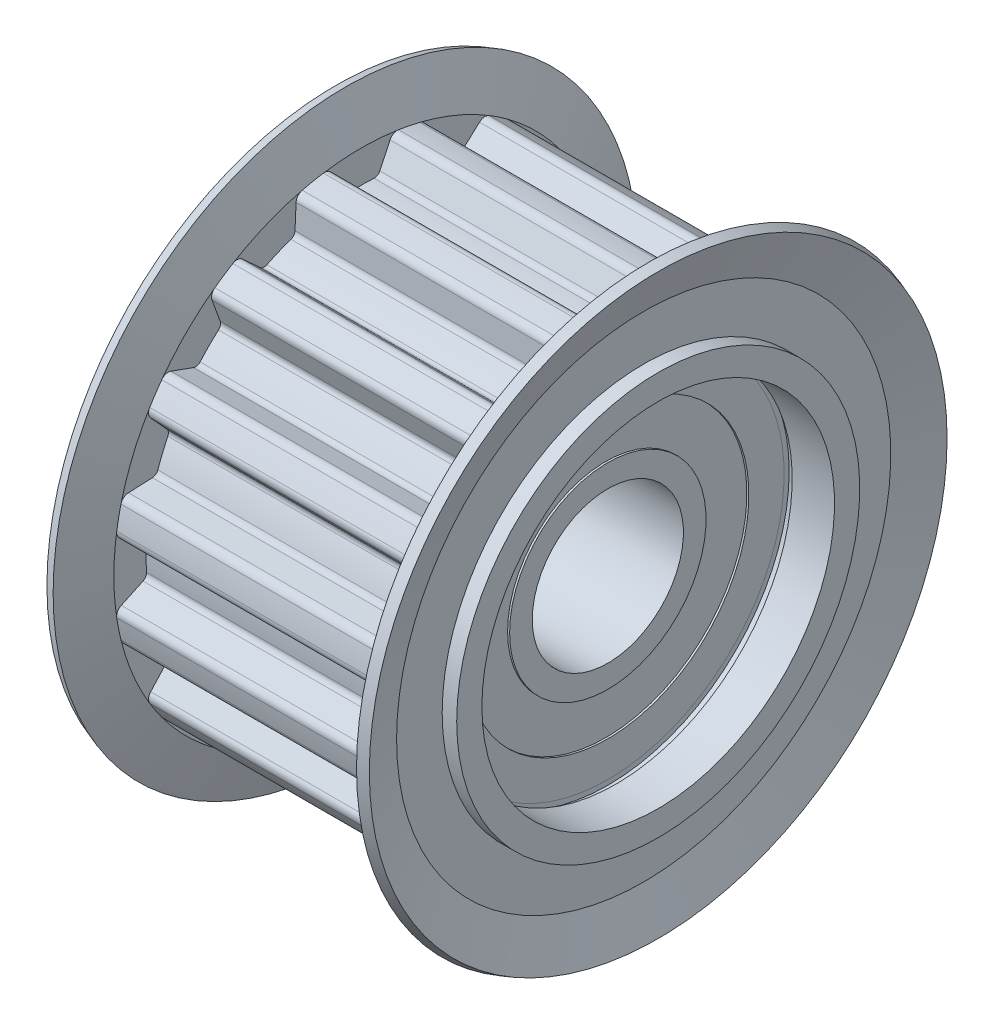
SolidWorks part; units mm, degrees
ref_plane "Front Plane" through (0, 0, 0) normal (0, 0, 1) x (1, 0, 0)
ref_plane "Top Plane" through (0, 0, 0) normal (0, 1, 0) x (1, 0, 0)
ref_plane "Right Plane" through (0, 0, 0) normal (1, 0, 0) x (0, 0, -1)
sketch "Sketch1" plane through (0, 0, 0) normal (0, 0, 1) x (1, 0, 0)
  line L0 (-68.412, 0) -> (82.0944, 0) construction
  line L1 (0, 75.1216) -> (0, -71.9641) construction
  line L2 (-16, 17) -> (-16, 20)
  line L3 (-16, 20) -> (-13.5, 20)
  line L4 (-13.5, 20) -> (-13.5, 24.525)
  line L5 (-13.5, 24.525) -> (13.5, 24.525)
  line L6 (13.5, 24.525) -> (13.5, 20)
  line L7 (13.5, 20) -> (16, 20)
  line L8 (16, 20) -> (16, 17.5)
  line L9 (-16, 17) -> (-11, 17)
  line L10 (-11, 17) -> (-11, 17.5)
  line L11 (-11, 17.5) -> (11, 17.5)
  line L12 (11, 17.5) -> (11, 18)
  line L13 (11, 18) -> (11.8, 18)
  line L14 (11.8, 18) -> (11.8, 17.5)
  line L15 (11.8, 17.5) -> (16, 17.5)
revolve "Revolve1" add sketch "Sketch1" angle 360 about L0
sketch "Sketch2" plane through (-13.5, 0, 0) normal (-1, 0, 0) x (0, 0, 1)
  line L0 (-7.5464, 0) -> (7.1688, 0) construction
  line L1 (0, 7.2233) -> (0, -7.4574) construction
  line L2 (-2.88, 23.7876) -> (-1.8743, 21.631)
  line L3 (2.88, 23.7876) -> (1.8743, 21.631)
  line L4 (-1.8743, 21.631) -> (-1.7, 21.2571) construction
  line L5 (1.8743, 21.631) -> (1.7, 21.2571) construction
  arc A0 (3.7266, 24.2402) -> (-3.7266, 24.2402) centre (0, 0) ccw
  arc A1 (1.2941, 21.2857) -> (-1.2941, 21.2857) centre (0, 0) ccw
  arc A2 (-3.7266, 24.2402) -> (-2.88, 23.7876) centre (-3.605, 23.4495) cw
  arc A3 (-1.8743, 21.631) -> (-1.2941, 21.2857) centre (-1.3306, 21.8846) ccw
  arc A4 (1.8743, 21.631) -> (1.2941, 21.2857) centre (1.3306, 21.8846) cw
  arc A5 (3.7266, 24.2402) -> (2.88, 23.7876) centre (3.605, 23.4495) ccw
extrude "Cut-Extrude1" cut sketch "Sketch2" against normal blind 32
ref_axis "Axis1" through (-8.7445, 0, 0) along (1, 0, 0)
pattern_circular "CirPattern1" count 16 over 360 about axis through (0, 0, 0) along (1, 0, 0) of "Cut-Extrude1"
sketch "Sketch3" plane through (0, 0, 0) normal (0, 0, 1) x (1, 0, 0)
  line L0 (-13.5, 20) -> (-13.5, 24.525)
  line L1 (-13.5, 24.525) -> (-15.0554, 29)
  line L2 (-15.0554, 29) -> (-16, 28.6717)
  line L3 (-16, 28.6717) -> (-14.5587, 24.525)
  line L4 (-14.5587, 24.525) -> (-14.5587, 20)
  line L5 (-14.5587, 20) -> (-13.5, 20)
  line L6 (-16, 20) -> (-16, -20) construction
revolve "Revolve2" add sketch "Sketch3" angle 360 about axis through (-8.7445, 0, 0) along (1, 0, 0)
sketch "Sketch4" plane through (0, 0, 0) normal (0, 0, 1) x (1, 0, 0)
  line L0 (13.5, 20) -> (13.5, 24.525)
  line L1 (13.5, 24.525) -> (15.0554, 29)
  line L2 (15.0554, 29) -> (16, 28.6717)
  line L3 (16, 28.6717) -> (14.5587, 24.525)
  line L4 (14.5587, 24.525) -> (14.5587, 20)
  line L5 (14.5587, 20) -> (13.5, 20)
  line L6 (16, -20) -> (16, 20) construction
revolve "Revolve3" add sketch "Sketch4" angle 360 about axis through (-8.7445, 0, 0) along (1, 0, 0)
sketch "Sketch5" plane through (0, 0, 0) normal (0, 0, 1) x (1, 0, 0)
  line L0 (-11, 7.5) -> (-11, 9.75)
  line L1 (-11, 9.75) -> (-10.8, 9.75)
  line L2 (-10.8, 9.75) -> (-10.8, 14)
  line L3 (-10.8, 14) -> (-11, 14)
  line L4 (-11, 14) -> (-11, 17.5)
  line L5 (-11, 17.5) -> (11, 17.5)
  line L6 (11, 17.5) -> (11, 14)
  line L7 (11, 14) -> (10.8, 14)
  line L8 (10.8, 14) -> (10.8, 9.75)
  line L9 (10.8, 9.75) -> (11, 9.75)
  line L10 (11, 9.75) -> (11, 7.5)
  line L11 (11, 7.5) -> (-11, 7.5)
  line L12 (0, -6.9046) -> (0, 7.3598) construction
revolve "Revolve5" add sketch "Sketch5" angle 360 about axis through (-8.7445, 0, 0) along (1, 0, 0)
sketch "Sketch6" plane through (-16, 0, 0) normal (-1, 0, 0) x (0, 0, 1)
  circle A0 centre (0, 0) radius 29
  circle A1 centre (0, 0) radius 42.5
extrude "Cut-Extrude2" [suppressed] cut sketch "Sketch6" against normal blind 32
equation "\"CS\"= 16"
equation "\"d\"= 15"
equation "\"PD\"= 50.93"
equation "\"OD\"= 49.05"
equation "\"F\"= 58"
equation "\"E\"= 40"
equation "\"A\"= 27"
equation "\"W\"= 32"
equation "\"S\"= 5"
equation "\"D1\"= 35"
equation "\"ZJG1\"= 0"
equation "\"QHP\"= 85"
equation "\"ZJG2\"= 0"
equation "\"ZJG3\"= 0"
equation "\"ZJG4\"= 0"
equation "\"D1@Sketch1\"=\"E\"/2"
equation "\"D2@Sketch1\"=\"OD\"/2"
equation "\"D3@Sketch1\"=\"A\""
equation "\"D4@Sketch1\"=\"W\""
equation "\"D2@Sketch2\"=\"OD\"/2"
equation "\"D1@Cut-Extrude1\"=\"W\""
equation "\"D1@CirPattern1\"=\"CS\""
equation "\"D1@Sketch3\"=\"E\"/2"
equation "\"D2@Sketch3\"=\"A\"/2"
equation "\"D3@Sketch3\"=\"OD\"/2"
equation "\"D4@Sketch3\"=\"F\"/2"
equation "\"D1@Sketch4\"=\"A\"/2"
equation "\"D2@Sketch4\"=\"E\"/2"
equation "\"D3@Sketch4\"=\"OD\"/2"
equation "\"D4@Sketch4\"=\"F\"/2"
equation "\"D6@Sketch1\"=\"S\""
equation "\"D10@Sketch1\"=\"D1\"/2"
equation "\"D2@Sketch5\"=\"d\"/2"
equation "\"D3@Sketch5\"=\"d\"*1.3/2"
equation "\"D4@Sketch5\"=\"D1\"*0.8/2"
equation "\"D5@Sketch5\"=\"D1\"/2"
equation "\"D1@Sketch6\"=\"F\""
equation "\"D2@Sketch6\"=\"QHP\""
equation "\"D1@Cut-Extrude2\"=\"W\""
equation "\"旋转2\"= IIF ( \"ZJG2\" = 1 , \"suppressed\" , if ( \"ZJG4\" = 1 , \"suppressed\" , \"unsuppressed\" ) )"
equation "\"旋转3\" = IIF ( \"ZJG2\" = 1 , \"suppressed\" , IIF ( \"ZJG3\" = 1 , \"suppressed\" , \"unsuppressed\" ) )"
equation "\"切除-拉伸2\"= IIF ( \"ZJG1\" = 1 , \"unsuppressed\" , \"suppressed\" )"
equation "\"D8@Sketch1\"=\"S\""
equation "\"D6@Sketch5\"=\"W\"-\"S\"*2"
equation "\"D1@Sketch2\"=\"OD\"/2-3.2"
